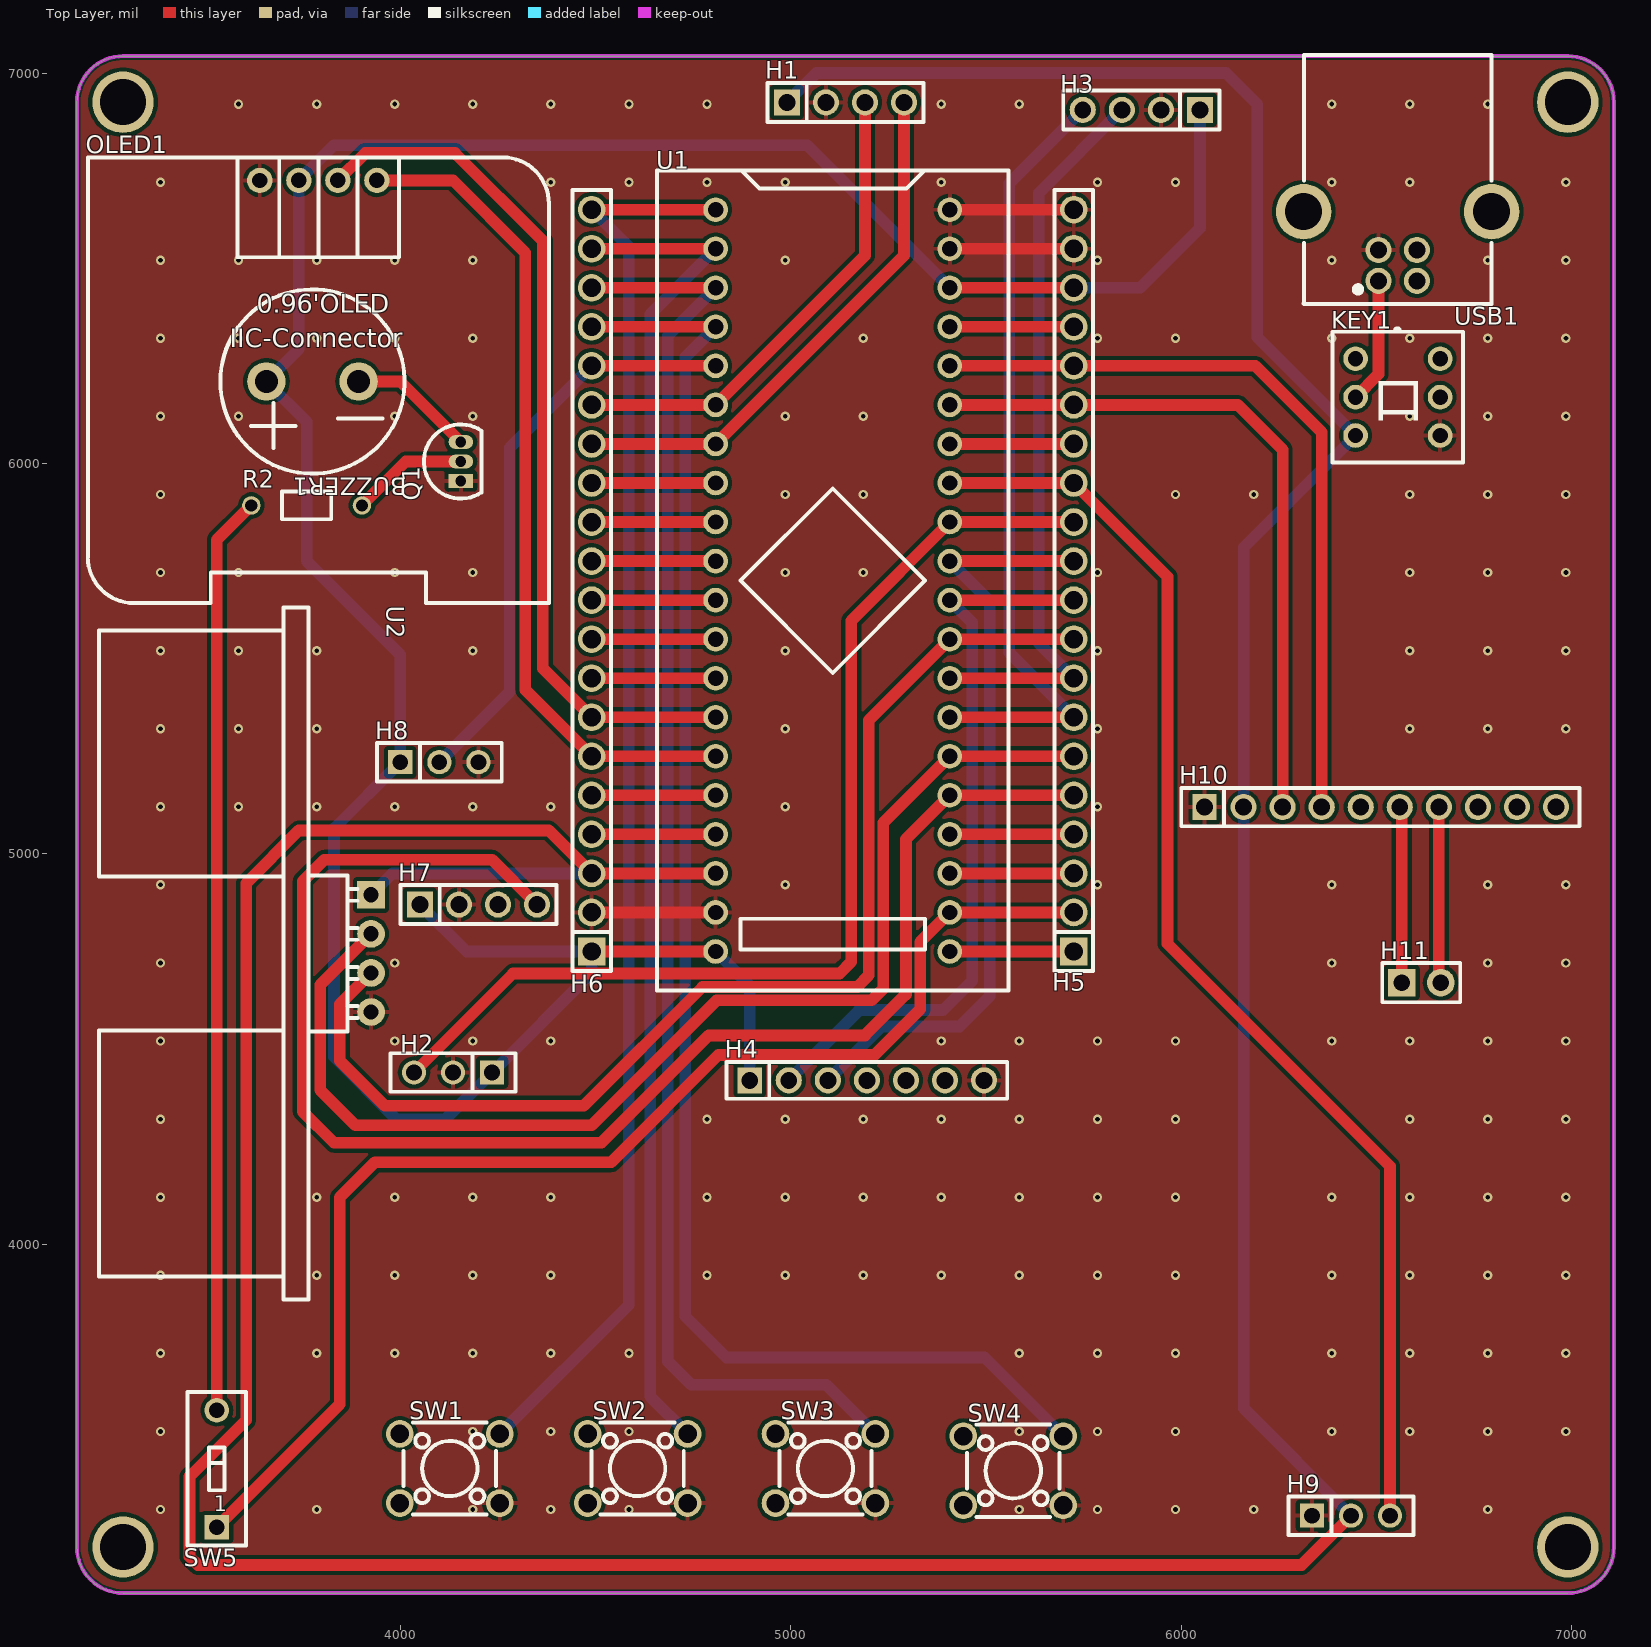
[diagram p0: Top Layer view]
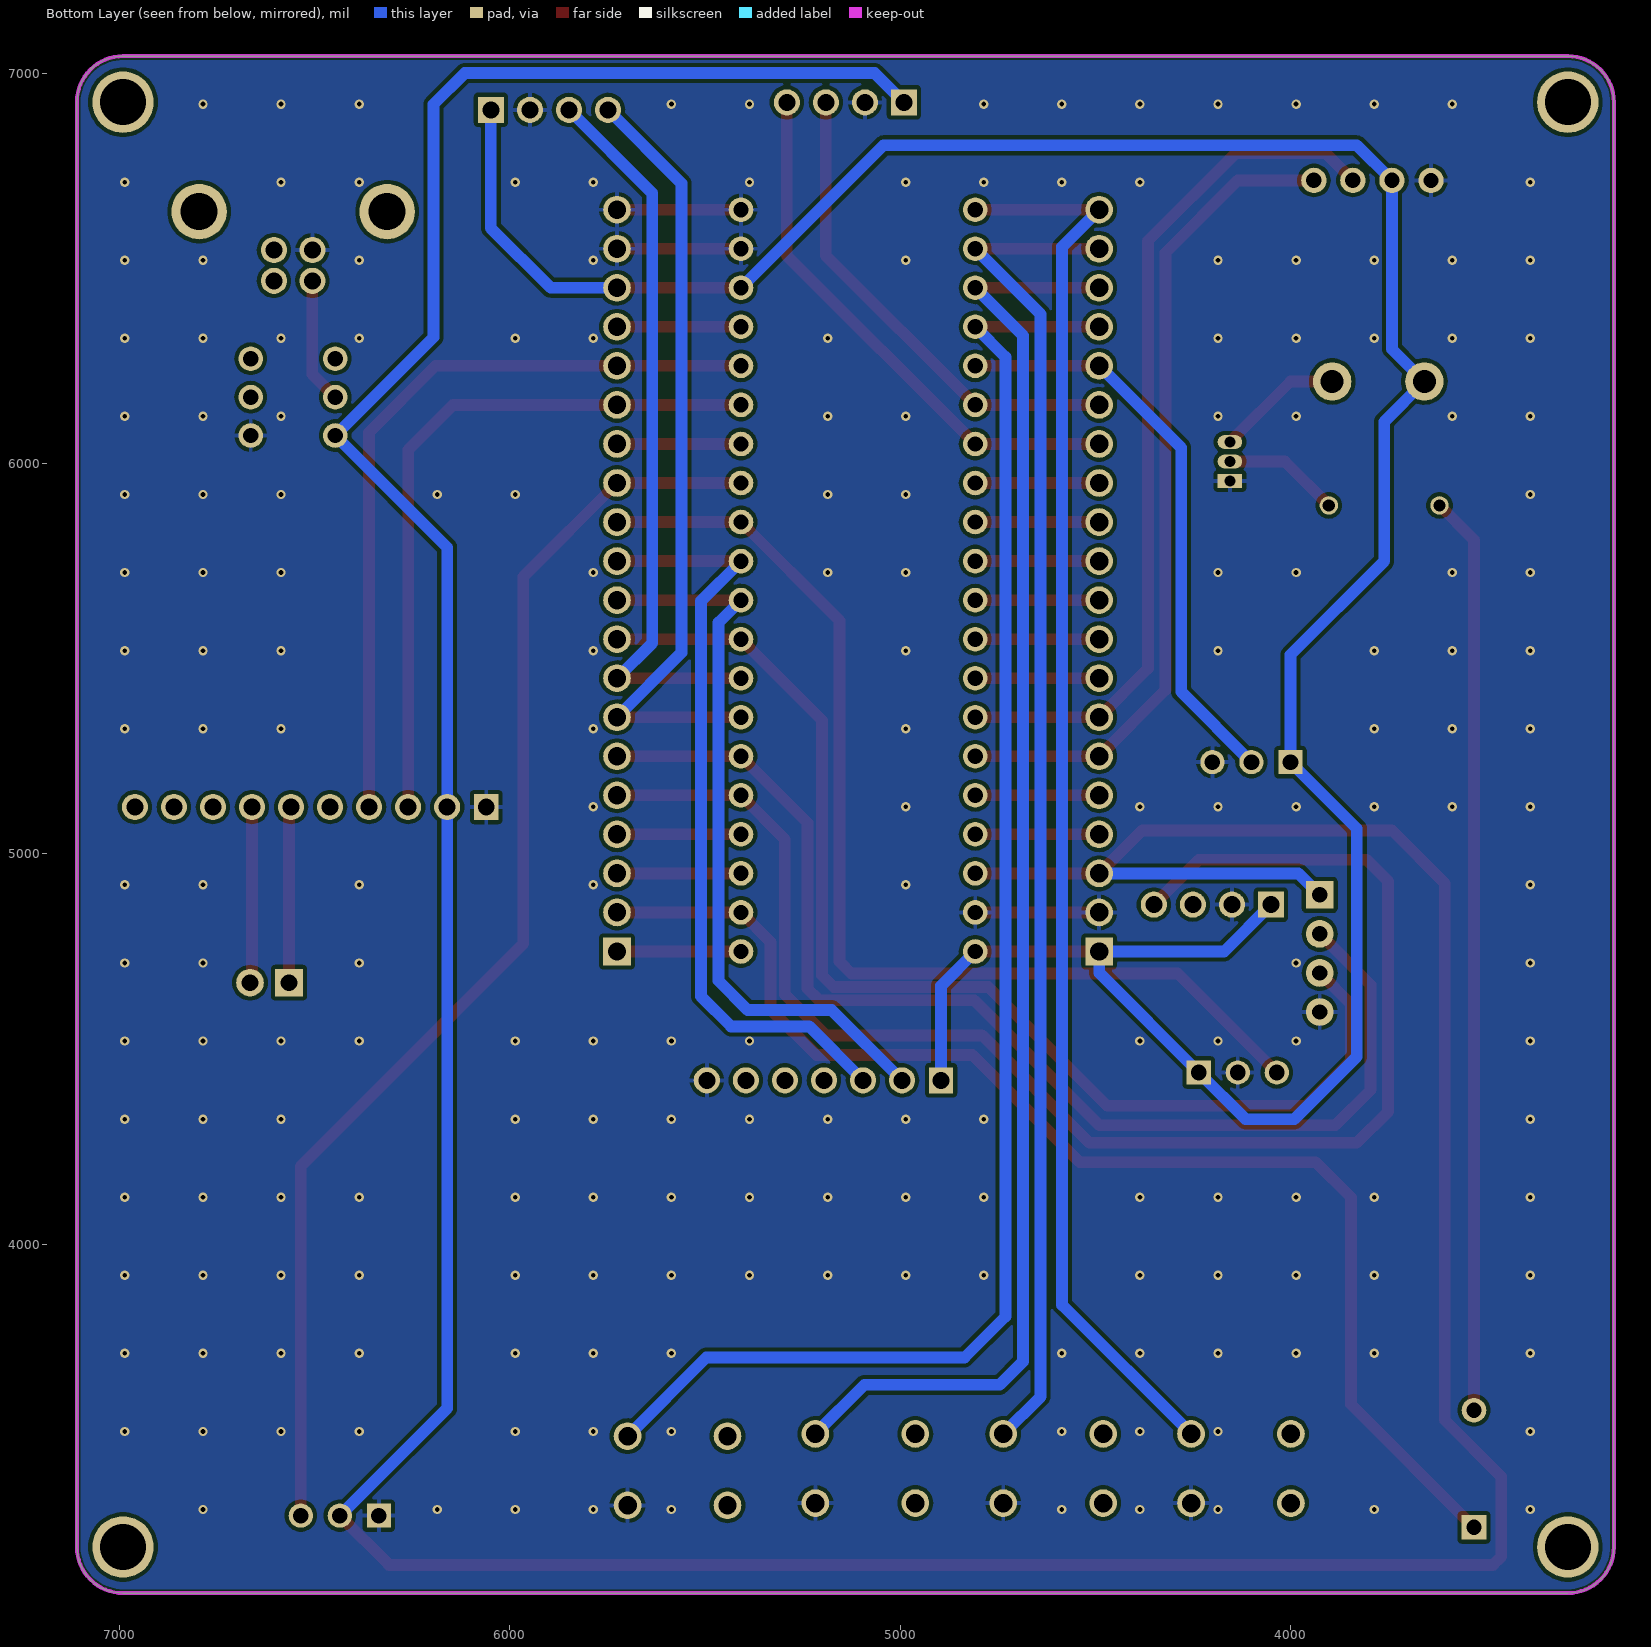
[diagram p1: Bottom Layer view, seen from below]
# Altium PCB MISC61230.pcbdoc
Units mil, origin at the board's own origin, x right, y up, seen from the top; angles counter-clockwise.
Board outline 3937.01 x 3937.01 mil, 2 copper layers (Top Layer, Bottom Layer), stack 62.206 mil thick; 24 components, 43 nets, 169 pads, 197 vias.

## Layer stack, top to bottom
Top Solder Mask Layer: solder mask 0.394, Dk 3.3
Top Layer: signal copper 1.379
Dielectric1: surface 59.449, FR4, Dk 4.5
Bottom Layer: signal copper 1.378
Bottom Solder Mask Layer: solder mask 0.394, Dk 3.3

## Board outline
6990.39,3106.5 ccw(c6990.39,3224.61) 7108.5,3224.61 7108.5,6925.39 ccw(c6990.39,6925.39) 6990.39,7043.5 3289.61,7043.5 ccw(c3289.61,6925.39) 3171.5,6925.39 3171.5,3224.61 ccw(c3289.61,3224.61) 3289.61,3106.5

## Design rules (kind name [scope] priority, off if disabled: settings)
BoardOutlineClearance copperThickness2oz_1 [All] p2 off: genericclearance=7.99 ignorepadtopadclearanceinfootprint=FALSE except(0: Arc-SplitContinuation Track-SplitContinuation SMDPad-SplitContinuation THPad-SplitContinuation Via-SplitContinuation Fill-SplitContinuation Region-SplitContinuation Poly-SplitContinuation Text-SplitContinuation Hole-SplitContinuation; 5.98: Arc-CutoutEdge Track-CutoutEdge SMDPad-CutoutEdge THPad-CutoutEdge Via-CutoutEdge Text-CutoutEdge; 6.89: Hole-OutlineEdge Hole-CutoutEdge; 10: Poly-OutlineEdge Poly-CutoutEdge; 11.81: Arc-OutlineEdge Track-OutlineEdge SMDPad-OutlineEdge THPad-OutlineEdge Via-OutlineEdge Fill-OutlineEdge Region-OutlineEdge Text-OutlineEdge Fill-CutoutEdge Region-CutoutEdge)
BoardOutlineClearance Plane_innerPlane_1 [All] p4 off: genericclearance=4.02 ignorepadtopadclearanceinfootprint=FALSE except(0: Arc-SplitContinuation Track-SplitContinuation SMDPad-SplitContinuation THPad-SplitContinuation Via-SplitContinuation Fill-SplitContinuation Region-SplitContinuation Poly-SplitContinuation Text-SplitContinuation Hole-SplitContinuation; 5.98: Arc-CutoutEdge Track-CutoutEdge SMDPad-CutoutEdge THPad-CutoutEdge Via-CutoutEdge Text-CutoutEdge; 6.89: Hole-OutlineEdge Hole-CutoutEdge; 10: Poly-OutlineEdge Poly-CutoutEdge; 11.81: Arc-OutlineEdge Track-OutlineEdge SMDPad-OutlineEdge THPad-OutlineEdge Via-OutlineEdge Fill-OutlineEdge Region-OutlineEdge Text-OutlineEdge Fill-CutoutEdge Region-CutoutEdge)
BoardOutlineClearance Copper_copperRegion_1 [All] p6 off: genericclearance=4.02 ignorepadtopadclearanceinfootprint=FALSE except(0: Arc-SplitContinuation Track-SplitContinuation SMDPad-SplitContinuation THPad-SplitContinuation Via-SplitContinuation Fill-SplitContinuation Region-SplitContinuation Poly-SplitContinuation Text-SplitContinuation Hole-SplitContinuation; 5.98: Arc-CutoutEdge Track-CutoutEdge SMDPad-CutoutEdge THPad-CutoutEdge Via-CutoutEdge Text-CutoutEdge; 6.89: Hole-OutlineEdge Hole-CutoutEdge; 10: Poly-OutlineEdge Poly-CutoutEdge; 11.81: Arc-OutlineEdge Track-OutlineEdge SMDPad-OutlineEdge THPad-OutlineEdge Via-OutlineEdge Fill-OutlineEdge Region-OutlineEdge Text-OutlineEdge Fill-CutoutEdge Region-CutoutEdge)
BoardOutlineClearance copperThickness1oz_1 [All] p8: genericclearance=4.02 ignorepadtopadclearanceinfootprint=FALSE except(0: Arc-SplitContinuation Track-SplitContinuation SMDPad-SplitContinuation THPad-SplitContinuation Via-SplitContinuation Fill-SplitContinuation Region-SplitContinuation Poly-SplitContinuation Text-SplitContinuation Hole-SplitContinuation; 5.98: Arc-CutoutEdge Track-CutoutEdge SMDPad-CutoutEdge THPad-CutoutEdge Via-CutoutEdge Text-CutoutEdge; 6.89: Hole-OutlineEdge Hole-CutoutEdge; 10: Poly-OutlineEdge Poly-CutoutEdge; 11.81: Arc-OutlineEdge Track-OutlineEdge SMDPad-OutlineEdge THPad-OutlineEdge Via-OutlineEdge Fill-OutlineEdge Region-OutlineEdge Text-OutlineEdge Fill-CutoutEdge Region-CutoutEdge)
Clearance copperThickness2oz [All] p1 off: gap=7.99 ignorepadtopadclearanceinfootprint=FALSE except(5.98: SMDPad-Track SMDPad-SMDPad THPad-Track SMDPad-THPad THPad-THPad Track-Via SMDPad-Via THPad-Via Via-Via Fill-SMDPad Region-SMDPad Fill-THPad Region-THPad Fill-Via Region-Via Fill-Fill Fill-Region Region-Region Arc-Track Arc-SMDPad Arc-THPad Arc-Via Fill-Arc Region-Arc Arc-Arc Text-Track SMDPad-Text Text-THPad Text-Via Fill-Text Region-Text Arc-Text Text-Text; 6.89: Hole-Track Hole-SMDPad Hole-THPad Hole-Via Fill-Hole Region-Hole Hole-Arc Hole-Text; 10: Poly-Track Poly-SMDPad Poly-THPad Poly-Via Poly-Fill Poly-Region Poly-Poly Poly-Arc Poly-Text Poly-Hole; 11.81: Fill-Track Region-Track)
Clearance Plane_innerPlane [All] p3 off: gap=4.02 ignorepadtopadclearanceinfootprint=FALSE except(5.98: SMDPad-Track SMDPad-SMDPad THPad-Track SMDPad-THPad THPad-THPad Track-Via SMDPad-Via THPad-Via Via-Via Fill-SMDPad Region-SMDPad Fill-THPad Region-THPad Fill-Via Region-Via Fill-Fill Fill-Region Region-Region Arc-Track Arc-SMDPad Arc-THPad Arc-Via Fill-Arc Region-Arc Arc-Arc Text-Track SMDPad-Text Text-THPad Text-Via Fill-Text Region-Text Arc-Text Text-Text; 6.89: Hole-Track Hole-SMDPad Hole-THPad Hole-Via Fill-Hole Region-Hole Hole-Arc Hole-Text; 10: Poly-Track Poly-SMDPad Poly-THPad Poly-Via Poly-Fill Poly-Region Poly-Poly Poly-Arc Poly-Text Poly-Hole; 11.81: Fill-Track Region-Track)
Clearance Copper_copperRegion [All] p5 off: gap=4.02 ignorepadtopadclearanceinfootprint=FALSE except(5.98: SMDPad-Track SMDPad-SMDPad THPad-Track SMDPad-THPad THPad-THPad Track-Via SMDPad-Via THPad-Via Via-Via Fill-SMDPad Region-SMDPad Fill-THPad Region-THPad Fill-Via Region-Via Fill-Fill Fill-Region Region-Region Arc-Track Arc-SMDPad Arc-THPad Arc-Via Fill-Arc Region-Arc Arc-Arc Text-Track SMDPad-Text Text-THPad Text-Via Fill-Text Region-Text Arc-Text Text-Text; 6.89: Hole-Track Hole-SMDPad Hole-THPad Hole-Via Fill-Hole Region-Hole Hole-Arc Hole-Text; 10: Poly-Track Poly-SMDPad Poly-THPad Poly-Via Poly-Fill Poly-Region Poly-Poly Poly-Arc Poly-Text Poly-Hole; 11.81: Fill-Track Region-Track)
Clearance copperThickness1oz [All] p7: gap=4.02 ignorepadtopadclearanceinfootprint=FALSE except(5.98: SMDPad-Track SMDPad-SMDPad THPad-Track SMDPad-THPad THPad-THPad Track-Via SMDPad-Via THPad-Via Via-Via Fill-SMDPad Region-SMDPad Fill-THPad Region-THPad Fill-Via Region-Via Fill-Fill Fill-Region Region-Region Arc-Track Arc-SMDPad Arc-THPad Arc-Via Fill-Arc Region-Arc Arc-Arc Text-Track SMDPad-Text Text-THPad Text-Via Fill-Text Region-Text Arc-Text Text-Text; 6.89: Hole-Track Hole-SMDPad Hole-THPad Hole-Via Fill-Hole Region-Hole Hole-Arc Hole-Text; 10: Poly-Track Poly-SMDPad Poly-THPad Poly-Via Poly-Fill Poly-Region Poly-Poly Poly-Arc Poly-Text Poly-Hole; 11.81: Fill-Track Region-Track)
DiffPairsRouting differentialPair [All] p1: maxlimit=6 minlimit=6 mostfreqgap=6 toplayer_minwidth=5 toplayer_prefwidth=10 toplayer_maxwidth=100 toplayer_mingap=6 toplayer_prefgap=6 toplayer_maxgap=6 bottomlayer_minwidth=5 bottomlayer_prefwidth=10 bottomlayer_maxwidth=100 bottomlayer_mingap=6 bottomlayer_prefgap=6 bottomlayer_maxgap=6 maxuncoupledlength=10
HoleToHoleClearance otherClearance [All] p1: gap=11.81 allowstackedmicrovias=TRUE
Length netLength [All] p1: minlimit=0 maxlimit=0
PasteMaskExpansion pasteMaskExpansion [All] p1: expansion=0
PlaneConnect innerPlane [All] p1: planeconnectstyle=Relief reliefexpansion=20 reliefentries=4 reliefconductorwidth=10 reliefairgap=10
PolygonConnect copperRegion [All] p1: connectstyle=Relief reliefconductorwidth=10 reliefentries=4 polygonreliefangle="90 Angle" airgapwidth=10 via.connectstyle=Relief via.reliefconductorwidth=10 via.reliefentries=4 via.polygonreliefangle="90 Angle" via.airgapwidth=10
RoutingVias viaSize [All] p1: holewidth=12.01 width=24.02 viastyle="Through Hole" minholewidth=11.81 minwidth=19.68 maxholewidth=248.03 maxwidth=393.7
SolderMaskExpansion solderMaskExpansion [IsVia] p1: expansion=-1000 istentingtop=TRUE
SolderMaskExpansion solderMaskExpansion [All] p2: expansion=2.01 istentingtop=FALSE
Width copperThickness2oz_2 [All] p1 off: maxlimit=100 minlimit=8 preferedwidth=10
Width copperThickness1oz_2 [All] p2: maxlimit=100 minlimit=5 preferedwidth=30

## Components (designator, comment, footprint, x,y, rotation, side; value= is the part's Value field where it differs from the comment)
BUZZER1 "buzzer" BUZ-TH_BD12.0-P6.00-D0.9-RD 3775,6210 r180 top
H1 "" HDR-TH_4P-P2.54-V-M 5140,6925 r0 top
H2 "" HDR-TH_3P-P2.54-V-F 4135,4440 r180 top
H3 "" HDR-TH_4P-P2.54-V-M 5898.05,6905.73 r180 top
H4 "" HDR-TH_7P-P2.54-V-F 5195,4420 r0 top
H5 "" HDR-TH_20P-P2.54-V-M-1 5725,5700 r90 top
H6 "" HDR-TH_20P-P2.54-V-M-1 4490,5700 r90 top
H7 "" HDR-TH_4P-P2.54-V-M 4200,4870 r0 top
H8 "" HDR-TH_3P-P2.54-V-F 4100,5235 r0 top
H9 "" HDR-TH_3P-P2.54-V-F 6435,3305 r0 top
H10 "" HDR-TH_10P-P2.54-V-F 6510,5120 r0 top
H11 "" HDR-TH_2P-P2.54-V-M-1 6615,4670 r0 top
KEY1 "Non-latching switch 8.5×8.5, silent" SW-TH_6P-L8.5-W8.5-P2.54 6555,6170 r270 top
OLED1 "" 0.96OLED_4P 3790,6725 r0 top
Q1 "" S8050_TO_92 4155,6005 r90 top
R2 "10kΩ" Res_1/8W 3760,5890 r0 top
SW1 "" SW-TH_4P-L6.0-W6.0-P4.50-LS6.5 4126.72,3425.65 r180 top
SW2 "" SW-TH_4P-L6.0-W6.0-P4.50-LS6.5 4607.81,3425.65 r180 top
SW3 "" SW-TH_4P-L6.0-W6.0-P4.50-LS6.5 5088.91,3425.65 r180 top
SW4 "" SW-TH_4P-L6.0-W6.0-P4.50-LS6.5 5570,3420 r180 top
SW5 "NDS-01V" SW-TH_2P-L3.9-W9.9-P2.54-LS7.6 3530,3425 r90 top
U1 "STM32F103C8T6-Card" CONN-TH_L53.3-W22.9_STM32F103C8T6-CARD 5107.5,5700 r270 top
U2 "HC-SR04" TH_HC-SR04V 3925,4745 r270 top
USB1 "" "USB_ Type-B" 6560,6725 r180 top

## Footprints (in the part's own frame and the unit in brackets; to place one, negate y for a bottom-side part, rotate by r counter-clockwise, add the part's x,y. Pads: shape width x height; smd on the part's side, far side on the other; paste and mask are expansions set on the pad)
0.96OLED_4P [mm]
  round 1.65 hole 1 copper offset 0,0: 1(-3.81,-0.001) 2(-1.27,0.002) 3(1.27,0.002) 4(3.81,0.002)
  silkscreen extent -15,-27.5 15,1.5
BUZ-TH_BD12.0-P6.00-D0.9-RD [mm]
  round 2.5 hole 1.5 paste+0 mask+0.05: 1(-3,0) 2(3,0)
  silkscreen extent -5.99,-5.99 5.99,5.99
CONN-TH_L53.3-W22.9_STM32F103C8T6-CARD [mm]
  round 1.6 hole 1: 1(-24.13,-7.62) 2(-21.59,-7.62) 3(-19.05,-7.62) 4(-16.51,-7.62) 5(-13.97,-7.62) 6(-11.43,-7.62) 7(-8.89,-7.62) 8(-6.35,-7.62) 9(-3.81,-7.62) 10(-1.27,-7.62) 11(1.27,-7.62) 12(3.81,-7.62) 13(6.35,-7.62) 14(8.89,-7.62) 15(11.43,-7.62) 16(13.97,-7.62) 17(16.51,-7.62) 18(19.05,-7.62) 19(21.59,-7.62) 20(24.13,-7.62) 21(24.13,7.62) 22(21.59,7.62) 23(19.05,7.62) 24(16.51,7.62) 25(13.97,7.62) 26(11.43,7.62) 27(8.89,7.62) 28(6.35,7.62) 29(3.81,7.62) 30(1.27,7.62) 31(-1.27,7.62) 32(-3.81,7.62) 33(-6.35,7.62) 34(-8.89,7.62) 35(-11.43,7.62) 36(-13.97,7.62) 37(-16.51,7.62) 38(-19.05,7.62) 39(-21.59,7.62) 40(-24.13,7.62)
  silkscreen extent -26.67,-11.43 26.67,11.43
HDR-TH_2P-P2.54-V-M-1 [mm]
  rect 1.8x1.8 hole 1.1: 1(-1.27,0)
  round 1.8 hole 1.1: 2(1.27,0)
  silkscreen extent -2.54,-1.27 2.54,1.27
HDR-TH_3P-P2.54-V-F [mil]
  rect 62x62 hole 40.16: 1(-100,0)
  round 62 hole 40.16: 2(0,0) 3(100,0)
  silkscreen extent -160,-49 160,49
HDR-TH_4P-P2.54-V-M [mm]
  rect 1.7x1.7 hole 1.1: 1(-3.81,0)
  round 1.7 hole 1.1: 2(-1.27,0) 3(1.27,0) 4(3.81,0)
  silkscreen extent -5.08,-1.27 5.08,1.27
HDR-TH_7P-P2.54-V-F [mm]
  rect 1.575x1.7 hole 1.1: 1(-7.62,0)
  round 1.7 hole 1.1: 2(-5.08,0) 3(-2.54,0) 4(0,0) 5(2.54,0) 6(5.08,0) 7(7.62,0)
  silkscreen extent -9.13,-1.2 9.13,1.2
HDR-TH_10P-P2.54-V-F [mm]
  rect 1.575x1.7 hole 1.1: 1(-11.43,0)
  round 1.7 hole 1.1: 2(-8.89,0) 3(-6.35,0) 4(-3.81,0) 5(-1.27,0) 6(1.27,0) 7(3.81,0) 8(6.35,0) 9(8.89,0) 10(11.43,0)
  silkscreen extent -12.95,-1.25 12.95,1.25
HDR-TH_20P-P2.54-V-M-1 [mm]
  rect 1.8x1.8 hole 1.2: 1(-24.13,0)
  round 1.8 hole 1.2: 2(-21.59,0) 3(-19.05,0) 4(-16.51,0) 5(-13.97,0) 6(-11.43,0) 7(-8.89,0) 8(-6.35,0) 9(-3.81,0) 10(-1.27,0) 11(1.27,0) 12(3.81,0) 13(6.35,0) 14(8.89,0) 15(11.43,0) 16(13.97,0) 17(16.51,0) 18(19.05,0) 19(21.59,0) 20(24.13,0)
  silkscreen extent -25.4,-1.25 25.4,1.25
Res_1/8W [mil]
  round 47.2 hole 31.5 paste+0 mask+2: 1(-141.7,2.48) 2(141.7,2.48)
  silkscreen extent -63,-33 63,38
S8050_TO_92 [mil]
  rect 35.4x63 hole 27.6 paste+0 mask+2: 1(-50,0)
  oval 35.4x63 hole 27.6 paste+0 mask+2: 2(0,0) 3(50,0)
  silkscreen extent -95,-53 95,95
SW-TH_2P-L3.9-W9.9-P2.54-LS7.6 [mm]
  rect 1.6x1.6 hole 1 paste+0 mask+0.05: 1(-3.81,0)
  round 1.6 hole 1 paste+0 mask+0.05: 2(3.81,0)
  silkscreen extent -5,-1.91 5,1.91
SW-TH_4P-L6.0-W6.0-P4.50-LS6.5 [mm]
  round 1.8 hole 1.2: 1(-3.25,2.25) 2(3.25,2.25) 3(-3.25,-2.25) 4(3.25,-2.25)
  silkscreen extent -3,-3 3,3
SW-TH_6P-L8.5-W8.5-P2.54 [mm]
  round 1.6 hole 1: 1(-2.5,-2.75) 2(0,-2.75) 3(2.5,-2.75) 4(-2.5,2.75) 5(0,2.75) 6(2.5,2.75)
  silkscreen extent -4.47,-4.25 4.25,4.25
TH_HC-SR04V [mm]
  rect 1.8x1.8 hole 1.001: 1(-3.81,0)
  round 1.8 hole 1.001: 2(-1.27,0) 3(1.27,0) 4(3.81,0)
  silkscreen extent -22.5,-17.7 22.5,-0.89
"USB_ Type-B" [mm]
  round 1.7 hole 1.1 copper offset 0,0 paste+0 mask+0.051: 1(1.39,6.532) 2(-1.11,6.532) 3(-1.11,4.532) 4(1.39,4.532)
  round 3.6 hole 2.4 paste+0 mask+0.051: 5(-5.977,2.032) 5(6.256,2.032)
  silkscreen extent -5.96,-8.17 6.25,8.03

## Free pads (board coordinates)
  round 157.48 hole 118.11: 1(3289.61,6925.39) 1(3289.61,3224.61) 1(6990.39,6925.39) 1(6990.39,3224.61)

## Via types
v1: diameter 24.02, hole 12, Top Layer to Bottom Layer, 197 vias

## Nets (pads, with @x,y where several pads share a name; then routed paths per layer and width w, separated by ;. In a path a pad name is that pad's centre, name@x,y a point inside that pad or via, vN(x,y) a via of type N, cw(c..) or ccw(c..) an arc to the next point about the centre after c; other vN are vias at no path point)
$1N18282: KEY1.2 USB1.1 | length 322.1
  Top Layer w30: KEY1.2 6505.29,6228.57 USB1.1
$1N18316: BUZZER1.1 Q1.3 | length 326.1
  Top Layer w30: BUZZER1.1 4000,6210 Q1.3
$1N18318: R2.1 SW5.2 | length 2354.1
  Top Layer w30: SW5.2 3530,5804.18 R2.1
$1N18319: Q1.2 R2.2 | length 299.9
  Top Layer w30: R2.2 4014.22,6005 Q1.2
$1N18345: H10.6 H11.1 | length 452.1
  Top Layer w30: H10.6 6565,5115 H11.1
$1N18346: H10.7 H11.2 | length 452.1
  Top Layer w30: H10.7 6660,4675 H11.2
+5V: H1.1 H6.3 H9.2 H10.2 KEY1.3 U1.18 U2.1 | length 11934
  Top Layer w30: U1.18 H6.3 4380,5060 3740,5060 3605,4925 3605,3550 3460,3405 3460,3200 3481.21,3178.79 6308.79,3178.79 H9.2
  Bottom Layer w30: U2.1 3980,4950 H6.3 ; H1.1 5065,7000 6115,7000 6195,6920 6195,6323.31 KEY1.3 6160,5784.85 H10.2 6160,3580 H9.2
GND: H1.2 H2.2 H3.2 H4.7 H5.19 H5.20 H6.2 H7.2 H8.3 H9.1 H10.1 KEY1.6 OLED1.1 Q1.1 SW1.1 SW2.1 SW3.1 SW4.1 U1.19 U1.39 U1.40 U2.4 USB1.4 | length 952.5
  Top Layer w30: H6.2 U1.19 ; U1.39 H5.19 ; U1.40 H5.20
  other v1: 3385.6,3320.6 3785.6,3320.6 4185.6,3320.6 4385.6,3320.6 4585.6,3320.6 5585.6,3320.6 5785.6,3320.6 5985.6,3320.6 6185.6,3320.6 6785.6,3320.6 3385.6,3520.6 4185.6,3520.6 4385.6,3520.6 4585.6,3520.6 5585.6,3520.6 5785.6,3520.6 5985.6,3520.6 6385.6,3520.6 6585.6,3520.6 6785.6,3520.6 6985.6,3520.6 3385.6,3720.6 3785.6,3720.6 3985.6,3720.6 4185.6,3720.6 4385.6,3720.6 4585.6,3720.6 5585.6,3720.6 5785.6,3720.6 5985.6,3720.6 6385.6,3720.6 6585.6,3720.6 6785.6,3720.6 6985.6,3720.6 3385.6,3920.6 3785.6,3920.6 3985.6,3920.6 4185.6,3920.6 4385.6,3920.6 4785.6,3920.6 4985.6,3920.6 5185.6,3920.6 5385.6,3920.6 5585.6,3920.6 5785.6,3920.6 5985.6,3920.6 6385.6,3920.6 6585.6,3920.6 6785.6,3920.6 6985.6,3920.6 3385.6,4120.6 3785.6,4120.6 3985.6,4120.6 4185.6,4120.6 4385.6,4120.6 4785.6,4120.6 4985.6,4120.6 5185.6,4120.6 5385.6,4120.6 5585.6,4120.6 5785.6,4120.6 5985.6,4120.6 6385.6,4120.6 6585.6,4120.6 6785.6,4120.6 6985.6,4120.6 3385.6,4320.6 4785.6,4320.6 4985.6,4320.6 5185.6,4320.6 5385.6,4320.6 5585.6,4320.6 5785.6,4320.6 5985.6,4320.6 6585.6,4320.6 6785.6,4320.6 6985.6,4320.6 3385.6,4520.6 3985.6,4520.6 4185.6,4520.6 4385.6,4520.6 5385.6,4520.6 5585.6,4520.6 5785.6,4520.6 5985.6,4520.6 6385.6,4520.6 6585.6,4520.6 6785.6,4520.6 6985.6,4520.6 3385.6,4720.6 3985.6,4720.6 6385.6,4720.6 6785.6,4720.6 6985.6,4720.6 3385.6,4920.6 4985.6,4920.6 5785.6,4920.6 6385.6,4920.6 6785.6,4920.6 6985.6,4920.6 3385.6,5120.6 3585.6,5120.6 3785.6,5120.6 3985.6,5120.6 4185.6,5120.6 4385.6,5120.6 4985.6,5120.6 5785.6,5120.6 3385.6,5320.6 3585.6,5320.6 3785.6,5320.6 4985.6,5320.6 5785.6,5320.6 6585.6,5320.6 6785.6,5320.6 6985.6,5320.6 3385.6,5520.6 3585.6,5520.6 3785.6,5520.6 4185.6,5520.6 4985.6,5520.6 5785.6,5520.6 6585.6,5520.6 6785.6,5520.6 6985.6,5520.6 3385.6,5720.6 3585.6,5720.6 3985.6,5720.6 4185.6,5720.6 4985.6,5720.6 5185.6,5720.6 5785.6,5720.6 6585.6,5720.6 6785.6,5720.6 6985.6,5720.6 3385.6,5920.6 4985.6,5920.6 5185.6,5920.6 5985.6,5920.6 6185.6,5920.6 6585.6,5920.6 6785.6,5920.6 6985.6,5920.6 3385.6,6120.6 3585.6,6120.6 3985.6,6120.6 4185.6,6120.6 4985.6,6120.6 5185.6,6120.6 6585.6,6120.6 6785.6,6120.6 6985.6,6120.6 3385.6,6320.6 3585.6,6320.6 3785.6,6320.6 3985.6,6320.6 4185.6,6320.6 5185.6,6320.6 5785.6,6320.6 5985.6,6320.6 6385.6,6320.6 6585.6,6320.6 6785.6,6320.6 6985.6,6320.6 3385.6,6520.6 3585.6,6520.6 3785.6,6520.6 3985.6,6520.6 4185.6,6520.6 4985.6,6520.6 5785.6,6520.6 6385.6,6520.6 6785.6,6520.6 6985.6,6520.6 3385.6,6720.6 4385.6,6720.6 4585.6,6720.6 4785.6,6720.6 4985.6,6720.6 5385.6,6720.6 5785.6,6720.6 5985.6,6720.6 6385.6,6720.6 6585.6,6720.6 6985.6,6720.6 3585.6,6920.6 3785.6,6920.6 3985.6,6920.6 4185.6,6920.6 4385.6,6920.6 4585.6,6920.6 4785.6,6920.6 5385.6,6920.6 5585.6,6920.6 6385.6,6920.6 6585.6,6920.6 6785.6,6920.6
NRST: H5.17 U1.37 | length 317.5
  Top Layer w30: U1.37 H5.17
PA0: H5.5 H7.4 U1.25 | length 3870.1
  Top Layer w30: H7.4 4235,4985 3805,4985 3750,4930 3750,4340 3830,4260 4515,4260 4790,4535 5190,4535 5295,4640 5295,5037.5 U1.25 H5.5
PA1: H5.6 U1.26 U2.2 | length 3061.2
  Top Layer w30: U2.2 3795,4665 3795,4395 3885,4305 4490,4305 4810,4625 5207.01,4625 5237.01,4655 5237.01,5079.51 U1.26 H5.6
PA2: H3.4 H5.7 U1.27 | length 2019.5
  Top Layer w30: U1.27 H5.7
  Bottom Layer w30: H5.7 5560,5515 5560,6717.68 H3.4
PA3: H3.3 H5.8 U1.28 | length 1898.8
  Top Layer w30: U1.28 H5.8
  Bottom Layer w30: H5.8 5635,5540 5635,6692.68 H3.3
PA4: H5.9 U1.29 U2.3 | length 3063.6
  Top Layer w30: U2.3 3845,4615 3845,4470 3960,4355 4470,4355 4774.02,4659.02 5170,4659.02 5200,4689.02 5200,5342.5 U1.29 H5.9
PA5: H4.2 H5.10 U1.30 | length 1891.9
  Top Layer w30: U1.30 H5.10
  Bottom Layer w30: H4.2 5175,4600 5390,4600 5465,4675 5465,5592.5 U1.30
PA6: H4.3 H5.11 U1.31 | length 1979
  Top Layer w30: U1.31 H5.11
  Bottom Layer w30: H4.3 5233.06,4558.06 5433.06,4558.06 5510,4635 5510,5647.5 U1.31
PA7: H2.3 H5.12 U1.32 | length 2786
  Top Layer w30: H2.3 4288.58,4693.58 5125,4693.58 5155,4723.58 5155,5597.5 U1.32 H5.12
PA8: H6.16 H8.2 U1.5 | length 1494
  Top Layer w30: H6.16 U1.5
  Bottom Layer w30: H8.2 4280,5415 4280,6040 H6.16
PA9: H1.3 H6.15 U1.6 | length 1250.9
  Top Layer w30: H6.15 U1.6 5190,6532.5 H1.3
PA10: H1.4 H6.14 U1.7 | length 1392.4
  Top Layer w30: H6.14 U1.7 5290,6532.5 H1.4
PA11: H6.13 U1.8 | length 317.5
  Top Layer w30: H6.13 U1.8
PA12: H6.12 U1.9 | length 317.5
  Top Layer w30: H6.12 U1.9
PA15: H6.11 U1.10 | length 317.5
  Top Layer w30: H6.11 U1.10
PB0: H5.13 H9.3 U1.33 | length 3298
  Top Layer w30: U1.33 H5.13 5965,5710 5965,4770 6535,4200 H9.3
PB1: H5.14 U1.34 | length 317.5
  Top Layer w30: U1.34 H5.14
PB3: H6.10 U1.11 | length 317.5
  Top Layer w30: H6.10 U1.11
PB4: H6.9 U1.12 | length 317.5
  Top Layer w30: H6.9 U1.12
PB5: H6.8 U1.13 | length 317.5
  Top Layer w30: H6.8 U1.13
PB6: H6.7 OLED1.3 U1.14 | length 2236.5
  Top Layer w30: OLED1.3@3840,6725.05 3909.95,6795 4140,6795 4365,6570 4365,5475 H6.7 U1.14
PB7: H6.6 OLED1.4 U1.15 | length 2134.6
  Top Layer w30: OLED1.4@3940,6725.05 4134.95,6725.05 4320,6540 4320,5420 H6.6 U1.15
PB8: H6.5 U1.16 | length 317.5
  Top Layer w30: H6.5 U1.16
PB9: H6.4 U1.17 | length 317.5
  Top Layer w30: H6.4 U1.17
PB10: H5.15 H10.3 U1.35 | length 1815.1
  Top Layer w30: U1.35 H5.15 6145,6150 6260,6035 H10.3
PB11: H5.16 H10.4 U1.36 | length 1982.9
  Top Layer w30: U1.36 H5.16 6190,6250 6360,6080 H10.4
PB12: H6.20 SW1.3 U1.1 | length 3629.4
  Top Layer w30: H6.20 U1.1
  Bottom Layer w30: SW1.3 4585,3844.56 4585,6555 H6.20
PB13: H6.19 SW2.3 U1.2 | length 3462.3
  Top Layer w30: H6.19 U1.2
  Bottom Layer w30: SW2.3 4640,3609.99 4640,6382.5 U1.2
PB14: H6.18 SW3.3 U1.3 | length 3727
  Top Layer w30: H6.18 U1.3
  Bottom Layer w30: U1.3 4685,6327.5 4685,3700 4745,3640 5091.09,3640 SW3.3
PB15: H6.17 SW4.3 U1.4 | length 3979.5
  Top Layer w30: H6.17 U1.4
  Bottom Layer w30: U1.4 4730,6272.5 4730,3815 4835,3710 5496.53,3710 SW4.3
PC13: H5.2 SW5.1 U1.22 | length 3258.9
  Top Layer w30: SW5.1 3845,3590 3845,4120 3935,4210 4540,4210 4815,4485 5215,4485 5332.05,4602.05 5332.05,4774.55 U1.22 H5.2
PC14: H5.3 U1.23 | length 317.5
  Top Layer w30: U1.23 H5.3
PC15: H5.4 U1.24 | length 317.5
  Top Layer w30: U1.24 H5.4
VBAT: H5.1 U1.21 | length 317.5
  Top Layer w30: U1.21 H5.1
VCC: BUZZER1.2 H2.1 H3.1 H4.1 H5.18 H6.1 H7.1 H8.1 OLED1.2 U1.20 U1.38 | length 7464.6
  Top Layer w30: H6.1 U1.20 ; U1.38 H5.18
  Bottom Layer w30: H7.1 4170,4750 H6.1 4490,4695 H2.1 4115,4320 3990,4320 3830,4480 3830,5065 H8.1 4000,5510 3760,5750 3760,6106.89 BUZZER1.2 3740,6293.11 3740,6725.05 3829.95,6815 5042.5,6815 U1.38 ; U1.20 4895,4662.5 H4.1 ; H5.18 5895,6450 6048.05,6603.05 H3.1
pads on no net: H4.4 H4.5 H4.6 H7.3 H10.5 H10.8 H10.9 H10.10 KEY1.1 KEY1.4 KEY1.5 SW1.2 SW1.4 SW2.2 SW2.4 SW3.2 SW3.4 SW4.2 SW4.4 USB1.2 USB1.3 USB1.5

## Polygon pours and split planes (outlines as drawn)
GND on Bottom Layer (solid, remove dead copper, pour order 2): 3100,7165 3100,3000 7275,3000 7275,7165
GND on Top Layer (solid, remove dead copper, pour order 0): 3000,7145 3000,3075 7385,3075 7385,7145

## Keep-outs
Board Outline Layer:
  the board outline again, w10